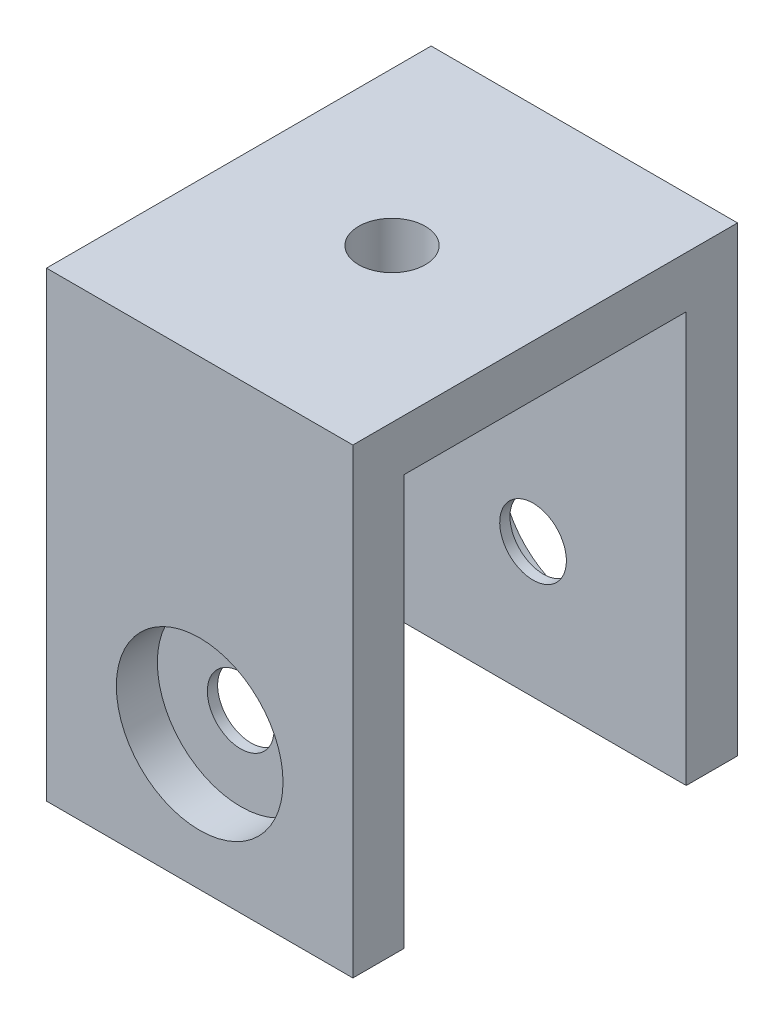
from build123d import *

# Parameters (mm, degrees)
SKETCH1_W           = 23.896551724
SKETCH1_H           = 25.5
BOSS_EXTRUDE1_DEPTH = 30
CUT_EXTRUDE1_DEPTH  = 41.417912914
SKETCH4_W           = 10
SKETCH4_H           = 5
CUT_EXTRUDE3_DEPTH  = 41.417912914
SKETCH7_W           = 6
SKETCH7_H           = 20
CUT_EXTRUDE4_DEPTH  = 23.896551724
SKETCH9_W           = 23.896551724
SKETCH9_H           = 30
BOSS_EXTRUDE3_DEPTH = 17.5
SKETCH12_W          = 23.896551724
SKETCH12_H          = 30
CUT_EXTRUDE7_DEPTH  = 8
SKETCH15_W          = 23.896551724
SKETCH15_H          = 30
CUT_EXTRUDE11_DEPTH = 6
SKETCH18_W          = 23.896551724
SKETCH18_H          = 4
BOSS_EXTRUDE4_DEPTH = 7
SKETCH19_W          = 30
SKETCH19_H          = 5
CUT_EXTRUDE12_DEPTH = 44.140557302
SKETCH20_R          = 2.6
CUT_EXTRUDE13_DEPTH = 45.763392366
SKETCH21_W          = 23.896551724
SKETCH21_H          = 4
BOSS_EXTRUDE5_DEPTH = 5
SKETCH22_R          = 2.6
CUT_EXTRUDE14_DEPTH = 41.685670648
SKETCH23_R          = 6.5
CUT_EXTRUDE15_DEPTH = 3.2


with BuildPart() as part:
    # Sketch1 → Boss-Extrude1 (new body)
    with BuildSketch(Plane.XY):
        Rectangle(SKETCH1_W, SKETCH1_H)
    extrude(amount=BOSS_EXTRUDE1_DEPTH)

    # Sketch2 → Cut-Extrude1 (cut, through all)
    with BuildSketch(Plane(origin=(11.948275862, 0, 0), x_dir=(0, 0, -1), z_dir=(1, 0, 0))):
        Polygon((-15, -12.75), (-20, -12.75), (-20, 2.25), (-10, 2.25), (-10, -12.75), align=None)
    extrude(amount=-CUT_EXTRUDE1_DEPTH, mode=Mode.SUBTRACT)

    # Sketch4 → Cut-Extrude3 (cut, through all)
    with BuildSketch(Plane(origin=(11.948275862, 0, 0), x_dir=(0, 0, -1), z_dir=(1, 0, 0))):
        with Locations((-15, 4.75)):
            Rectangle(SKETCH4_W, SKETCH4_H)
    extrude(amount=-CUT_EXTRUDE3_DEPTH, mode=Mode.SUBTRACT)

    # Sketch7 → Cut-Extrude4 (cut)
    with BuildSketch(Plane.ZY.offset(11.948275862)):
        with Locations((7, -2.75)):
            Rectangle(SKETCH7_W, SKETCH7_H)
        with Locations((23, -2.75)):
            Rectangle(SKETCH7_W, SKETCH7_H)
    extrude(amount=-CUT_EXTRUDE4_DEPTH, mode=Mode.SUBTRACT)

    # Sketch9 → Boss-Extrude3 (add)
    with BuildSketch(Plane(origin=(0, 12.75, 0), x_dir=(1, 0, 0), z_dir=(0, 1, 0))):
        with Locations((0, -15)):
            Rectangle(SKETCH9_W, SKETCH9_H)
    extrude(amount=BOSS_EXTRUDE3_DEPTH)

    # Sketch12 → Cut-Extrude7 (cut)
    with BuildSketch(Plane(origin=(0, 30.25, 0), x_dir=(1, 0, 0), z_dir=(0, 1, 0))):
        with Locations((0, -15)):
            Rectangle(SKETCH12_W, SKETCH12_H)
    extrude(amount=-CUT_EXTRUDE7_DEPTH, mode=Mode.SUBTRACT)

    # Sketch15 → Cut-Extrude11 (cut)
    with BuildSketch(Plane(origin=(0, 22.25, 0), x_dir=(1, 0, 0), z_dir=(0, 1, 0))):
        with Locations((0, -15)):
            Rectangle(SKETCH15_W, SKETCH15_H)
    extrude(amount=-CUT_EXTRUDE11_DEPTH, mode=Mode.SUBTRACT)

    # Sketch18 → Boss-Extrude4 (add)
    with BuildSketch(Plane.XZ.offset(12.75)):
        with Locations((0, 28)):
            Rectangle(SKETCH18_W, SKETCH18_H)
        with Locations((0, 2)):
            Rectangle(SKETCH18_W, SKETCH18_H)
    extrude(amount=BOSS_EXTRUDE4_DEPTH)

    # Sketch19 → Cut-Extrude12 (cut, through all)
    with BuildSketch(Plane(origin=(11.948275862, 0, 0), x_dir=(0, 0, -1), z_dir=(1, 0, 0))):
        with Locations((-15, 13.75)):
            Rectangle(SKETCH19_W, SKETCH19_H)
    extrude(amount=-CUT_EXTRUDE12_DEPTH, mode=Mode.SUBTRACT)

    # Sketch20 → Cut-Extrude13 (cut, through all)
    with BuildSketch(Plane(origin=(0, 11.25, 0), x_dir=(1, 0, 0), z_dir=(0, 1, 0))):
        with Locations(Location((0, -15, 0), (0, 0, 270))):
            Circle(SKETCH20_R)
    extrude(amount=-CUT_EXTRUDE13_DEPTH, mode=Mode.SUBTRACT)

    # Sketch21 → Boss-Extrude5 (add)
    with BuildSketch(Plane.XZ.offset(19.75)):
        with Locations((0, 2)):
            Rectangle(SKETCH21_W, SKETCH21_H)
        with Locations((0, 28)):
            Rectangle(SKETCH21_W, SKETCH21_H)
    extrude(amount=BOSS_EXTRUDE5_DEPTH)

    # Sketch22 → Cut-Extrude14 (cut, through all)
    with BuildSketch(Plane.XY.offset(30)):
        with Locations((0, -14.25)):
            Circle(SKETCH22_R)
    extrude(amount=-CUT_EXTRUDE14_DEPTH, mode=Mode.SUBTRACT)

    # Sketch23 → Cut-Extrude15 (cut)
    with BuildSketch(Plane(origin=(0, 0, 0), x_dir=(-1, 0, 0), z_dir=(0, 0, -1))):
        with Locations((0, -14.25)):
            Circle(SKETCH23_R)
    cut_extrude15 = extrude(amount=-CUT_EXTRUDE15_DEPTH, mode=Mode.SUBTRACT)

    # Mirror1: Cut-Extrude15 across plane
    add(cut_extrude15.mirror(Plane(origin=(0, 0, 15), x_dir=(1, 0, 0), z_dir=(0, 0, -1))), mode=Mode.SUBTRACT)


solid = part.part
